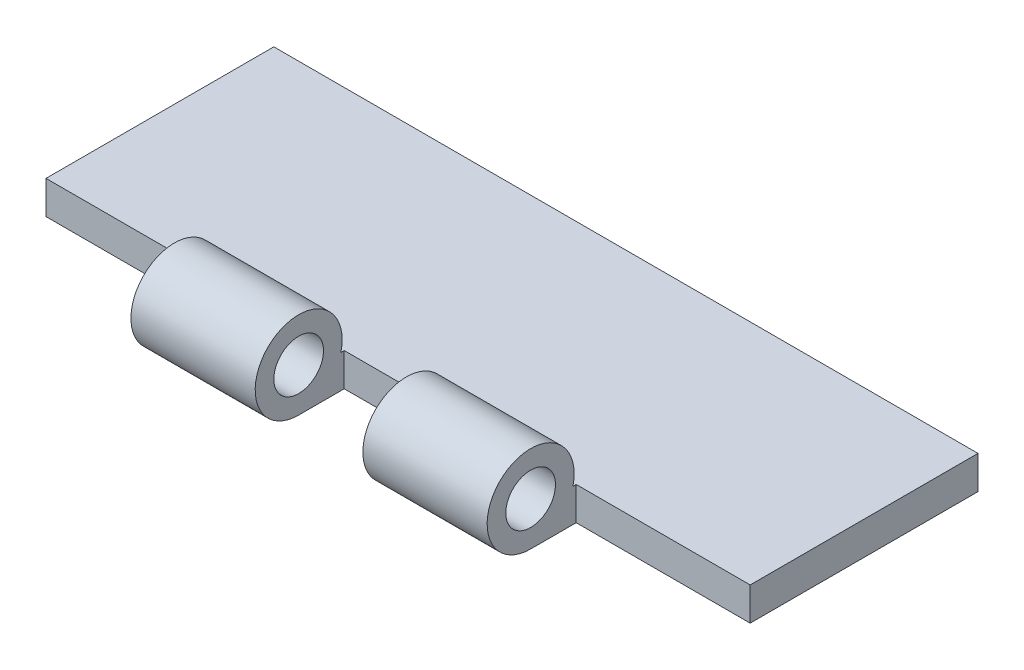
from build123d import *

# Parameters (mm, degrees)
BOSS_EXTRUDE1_DEPTH = 42.5
SKETCH3_W           = 13
SKETCH3_H           = 11
SKETCH3_W_2         = 21
SKETCH3_H_2         = 10.75
CUT_EXTRUDE2_DEPTH  = 10
SKETCH4_R           = 3
CUT_EXTRUDE3_DEPTH  = 73.198078229


with BuildPart() as part:
    # Sketch1 → Boss-Extrude1 (new, symmetric)
    with BuildSketch(Plane(origin=(0, 0, 0), x_dir=(0, 0, -1), z_dir=(1, 0, 0))):
        with BuildLine():
            Line((33, -5.25), (0, -5.25))
            ThreePointArc((0, -5.25), (-3.240370349, 4.13067791), (5.099019514, -1.25))
            Line((5.099019514, -1.25), (33, -1.25))
            Line((33, -1.25), (33, -5.25))
        make_face()
    extrude(amount=BOSS_EXTRUDE1_DEPTH, both=True)

    # Sketch3 → Cut-Extrude2 (cut, symmetric)
    with BuildSketch(Plane(origin=(0, 0, 0), x_dir=(1, 0, 0), z_dir=(0, 1, 0))):
        Rectangle(SKETCH3_W, SKETCH3_H)
        with Locations((32, 0.125)):
            Rectangle(SKETCH3_W_2, SKETCH3_H_2)
        with Locations((-32, 0.125)):
            Rectangle(SKETCH3_W_2, SKETCH3_H_2)
    extrude(amount=CUT_EXTRUDE2_DEPTH, both=True, mode=Mode.SUBTRACT)

    # Sketch4 → Cut-Extrude3 (cut, through all)
    with BuildSketch(Plane.ZY.offset(21.5)):
        Circle(SKETCH4_R)
    extrude(amount=-CUT_EXTRUDE3_DEPTH, mode=Mode.SUBTRACT)


solid = part.part
